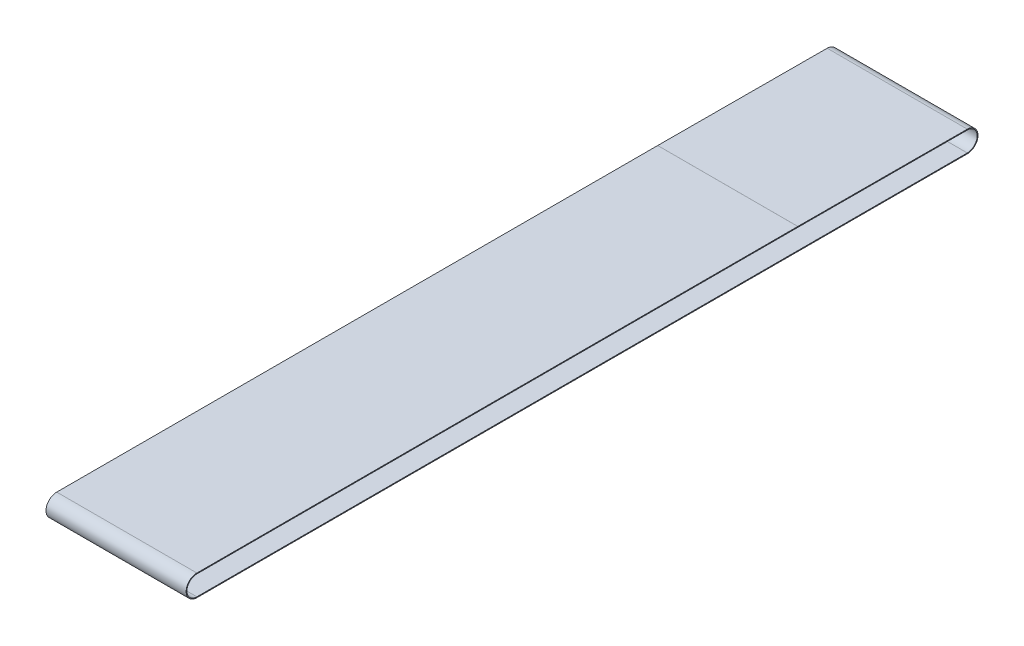
from build123d import *

# Parameters (mm, degrees)
EXTRUDE_1_DEPTH = 850


with BuildPart() as part:
    # 草图1 → 凸台-拉伸1 (new body)
    with BuildSketch(Plane(origin=(421.4, 0, 0), x_dir=(0, 0, -1), z_dir=(1, 0, 0))):
        with BuildLine():
            Line((-393.96433471, -99.400009785), (3251.03566529, -101.400009785))
            ThreePointArc((3251.03566529, -101.400009785), (3251.112676678, -101.400097662), (3251.189687908, -101.400276781))
            Line((3251.189687908, -101.400276781), (4279.189687908, -104.400276781))
            ThreePointArc((4279.189687908, -104.400276781), (4343.999870762, -169.529618225), (4278.93045157, -234.399962792))
            Line((4278.93045157, -234.399962792), (-394.06954843, -229.399962792))
            ThreePointArc((-394.06954843, -229.399962792), (-458.999978712, -164.347393138), (-393.96433471, -99.400009785))
        make_face()
        with BuildLine():
            Line((-393.967078194, -104.400009032), (3251.032921806, -106.400009032))
            ThreePointArc((3251.032921806, -106.400009032), (3251.104009241, -106.400090149), (3251.175096531, -106.400255491))
            Line((3251.175096531, -106.400255491), (4279.175096531, -109.400255491))
            ThreePointArc((4279.175096531, -109.400255491), (4338.999880704, -169.519647592), (4278.935801449, -229.399965655))
            Line((4278.935801449, -229.399965655), (-394.064198551, -224.399965655))
            ThreePointArc((-394.064198551, -224.399965655), (-453.999980349, -164.35143982), (-393.967078194, -104.400009032))
        make_face(mode=Mode.SUBTRACT)
    extrude(amount=-EXTRUDE_1_DEPTH)


solid = part.part
